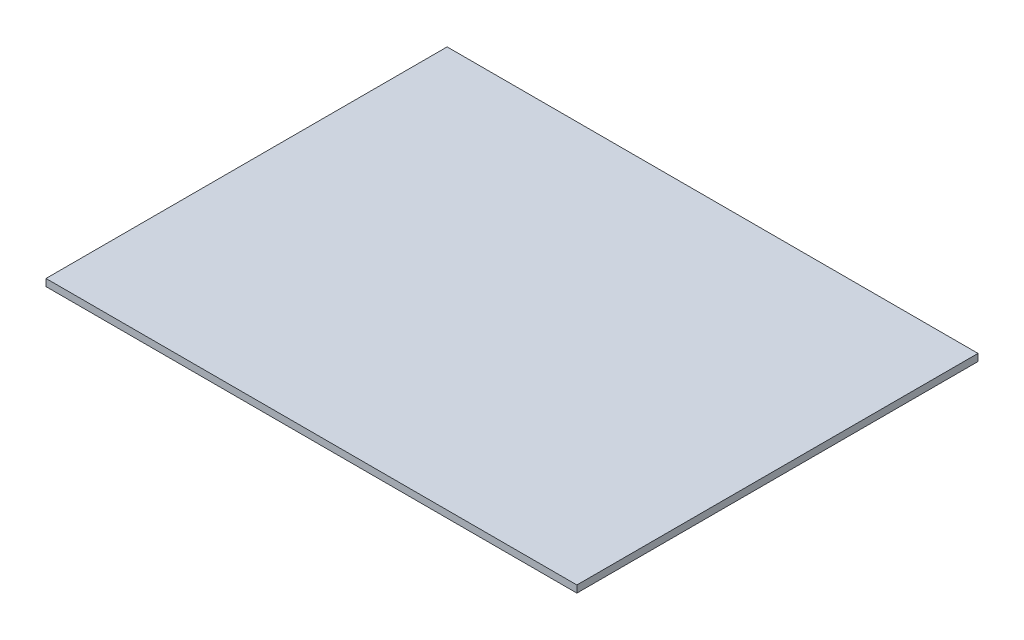
SolidWorks part; units mm, degrees
ref_plane "Front Plane" through (0, 0, 0) normal (0, 0, 1) x (1, 0, 0)
ref_plane "Top Plane" through (0, 0, 0) normal (0, 1, 0) x (1, 0, 0)
ref_plane "Right Plane" through (0, 0, 0) normal (1, 0, 0) x (0, 0, -1)
ref_plane "Plane1" through (0, -5, 0) normal (0, 1, 0) x (1, 0, 0)
sketch "Sketch1" plane through (0, -5, 0) normal (0, 1, 0) x (1, 0, 0)
  line L0 (50, 60) -> (500, 60)
  line L1 (500, 60) -> (500, 400)
  line L2 (500, 400) -> (50, 400)
  line L3 (50, 400) -> (50, 60)
extrude "Boss-Extrude1" add sketch "Sketch1" against normal blind 6
